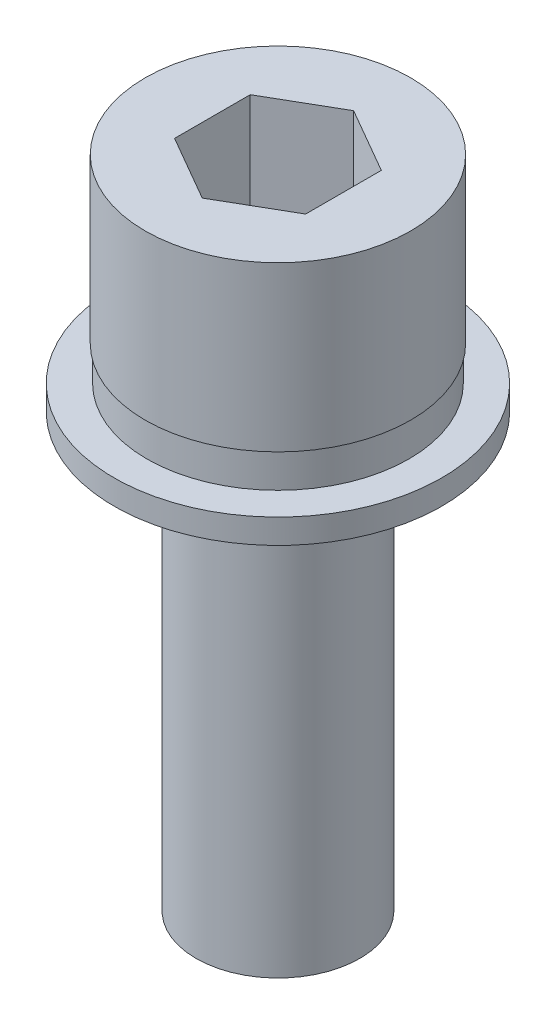
from build123d import *

# Parameters (mm, degrees)
CUT_EXTRUDE_1_DEPTH  = 6
SKETCH_3_R           = 8
SKETCH_3_R_2         = 5
BOSS_EXTRUDE_1_DEPTH = 2.1
SKETCH_4_R           = 10
SKETCH_4_R_2         = 5
BOSS_EXTRUDE_2_DEPTH = 1.5


with BuildPart() as part:
    # Sketch 1 → Revolve 1 (revolve)
    with BuildSketch(Plane.XY, mode=Mode.PRIVATE) as revolve_1_sk:
        Polygon((0, 10), (-8.1, 10), (-8.1, 0), (-5, 0), (-5, -30), (0, -30), align=None)
    revolve(revolve_1_sk.sketch.rotate(Axis((0, 11.322033898, 0), (0, -1, 0)), 270), axis=Axis((0, 11.322033898, 0), (0, -1, 0)))

    # Sketch 2 → Cut-Extrude 1 (cut)
    with BuildSketch(Plane(origin=(0, 10, 0), x_dir=(1, 0, 0), z_dir=(0, 1, 0))):
        Polygon((0, 4.618802154), (-4, 2.309401077), (-4, -2.309401077), (0, -4.618802154), (4, -2.309401077), (4, 2.309401077), align=None)
    extrude(amount=-CUT_EXTRUDE_1_DEPTH, mode=Mode.SUBTRACT)


with BuildPart() as body_2:
    # Sketch 3 → Boss-Extrude 1 (new body)
    with BuildSketch(Plane.XZ):
        with Locations(Location((0, 0, 0), (0, 0, 270))):
            Circle(SKETCH_3_R)
        with Locations(Location((0, 0, 0), (0, 0, 270))):
            Circle(SKETCH_3_R_2, mode=Mode.SUBTRACT)
    extrude(amount=BOSS_EXTRUDE_1_DEPTH)


with BuildPart() as body_3:
    # Sketch 4 → Boss-Extrude 2 (new body)
    with BuildSketch(Plane.XZ.offset(2.1)):
        with Locations(Location((0, 0, 0), (0, 0, 270))):
            Circle(SKETCH_4_R)
        with Locations(Location((0, 0, 0), (0, 0, 270))):
            Circle(SKETCH_4_R_2, mode=Mode.SUBTRACT)
    extrude(amount=BOSS_EXTRUDE_2_DEPTH)


solid = Compound([part.part, body_2.part, body_3.part])
